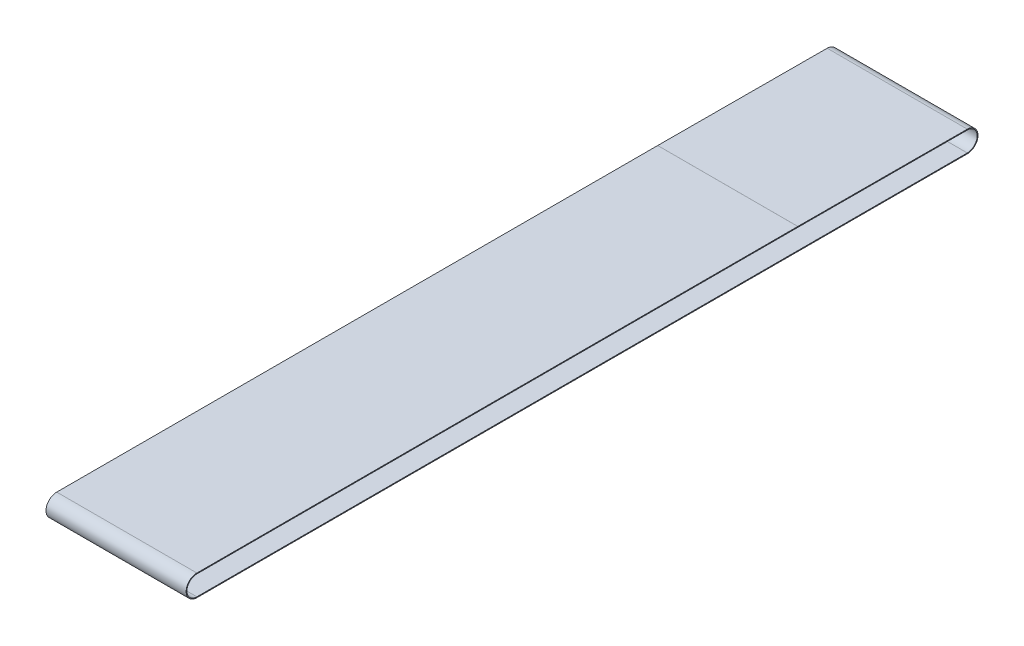
SolidWorks part; units mm, degrees
ref_plane "前视基准面" through (0, 0, 0) normal (0, 0, 1) x (1, 0, 0)
ref_plane "上视基准面" through (0, 0, 0) normal (0, 1, 0) x (1, 0, 0)
ref_plane "右视基准面" through (0, 0, 0) normal (1, 0, 0) x (0, 0, -1)
sketch "草图1" plane through (421.4, 0, 0) normal (1, 0, 0) x (0, 0, -1)
  line L0 (-393.9671, -104.4) -> (3251.0329, -106.4)
  line L1 (-394.0642, -224.4) -> (4278.9358, -229.4)
  line L2 (3251.1751, -106.4003) -> (4279.1751, -109.4003)
  line L3 (-393.9643, -99.4) -> (3251.0357, -101.4)
  line L4 (3251.1897, -101.4003) -> (4279.1897, -104.4003)
  line L5 (-394.0695, -229.4) -> (4278.9305, -234.4)
  arc A0 (3251.1897, -101.4003) -> (3251.0357, -101.4) centre (3251, -166.4) ccw
  circle A1 centre (-394, -164.4) radius 60
  arc A2 (-393.9671, -104.4) -> (-394.0642, -224.4) centre (-394, -164.4) ccw
  circle A3 centre (3251, -166.4) radius 60
  arc A4 (3251.1751, -106.4003) -> (3251.0329, -106.4) centre (3251, -166.4) ccw
  circle A5 centre (4279, -169.4) radius 60
  arc A6 (4278.9358, -229.4) -> (4279.1751, -109.4003) centre (4279, -169.4) ccw
  arc A7 (4278.9305, -234.4) -> (4279.1897, -104.4003) centre (4279, -169.4) ccw
  arc A8 (-393.9643, -99.4) -> (-394.0695, -229.4) centre (-394, -164.4) ccw
  dimension "D4" = 5
  dimension "D1" = 0
  dimension "D2" = 0
  dimension "D3" = 0
extrude "凸台-拉伸1" add sketch "草图1" against normal up to surface (850 mm away)
